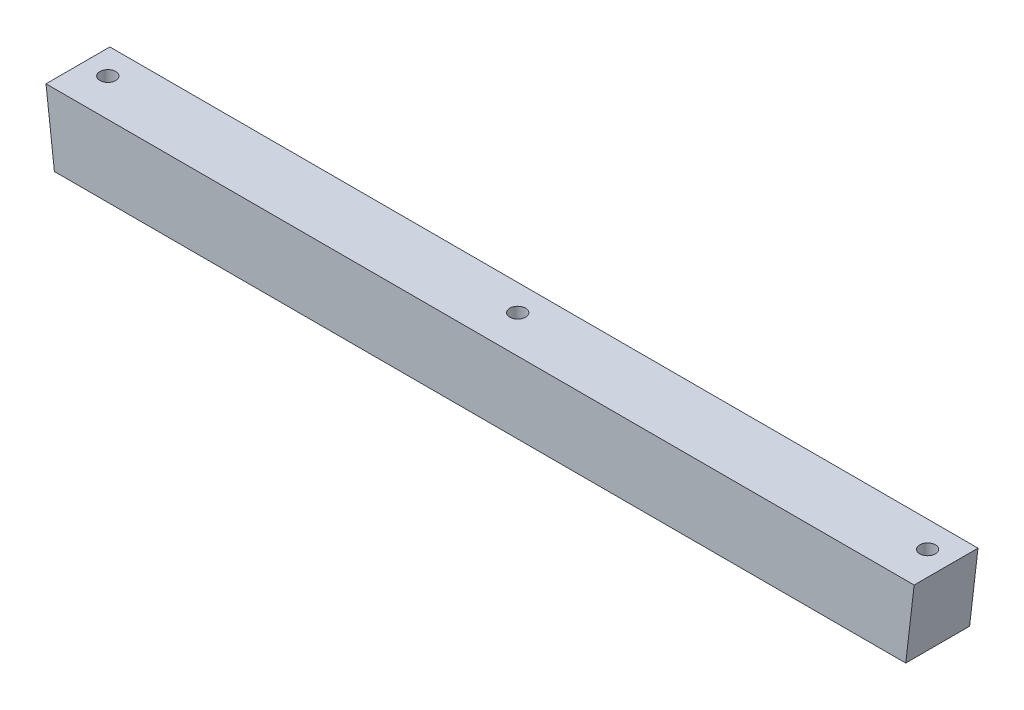
SolidWorks part; units mm, degrees
ref_plane "前视基准面" through (0, 0, 0) normal (0, 0, 1) x (1, 0, 0)
ref_plane "上视基准面" through (0, 0, 0) normal (0, 1, 0) x (1, 0, 0)
ref_plane "右视基准面" through (0, 0, 0) normal (1, 0, 0) x (0, 0, -1)
sketch "草图1" plane through (0, 0, 0) normal (0, 0, 1) x (1, 0, 0)
  line L0 (0, 0) -> (550.66, 0)
  line L2 (275.33, -45.55) -> (545.33, -45.55)
  line L4 (275.33, -45.55) -> (5.33, -45.55)
  line L6 (0, 0) -> (5.33, -45.55)
  line L7 (550.66, 0) -> (545.33, -45.55)
extrude "凸台-拉伸1" add sketch "草图1" along normal mid plane 40.5
sketch "草图2" plane through (0, 0, 0) normal (0, 1, 0) x (1, 0, 0)
  circle A0 centre (535.33, 3.62) radius 5
  circle A1 centre (275.33, 3.62) radius 5
  circle A2 centre (15.33, 3.62) radius 5
extrude "切除-拉伸1" cut sketch "草图2" against normal blind 52.5
